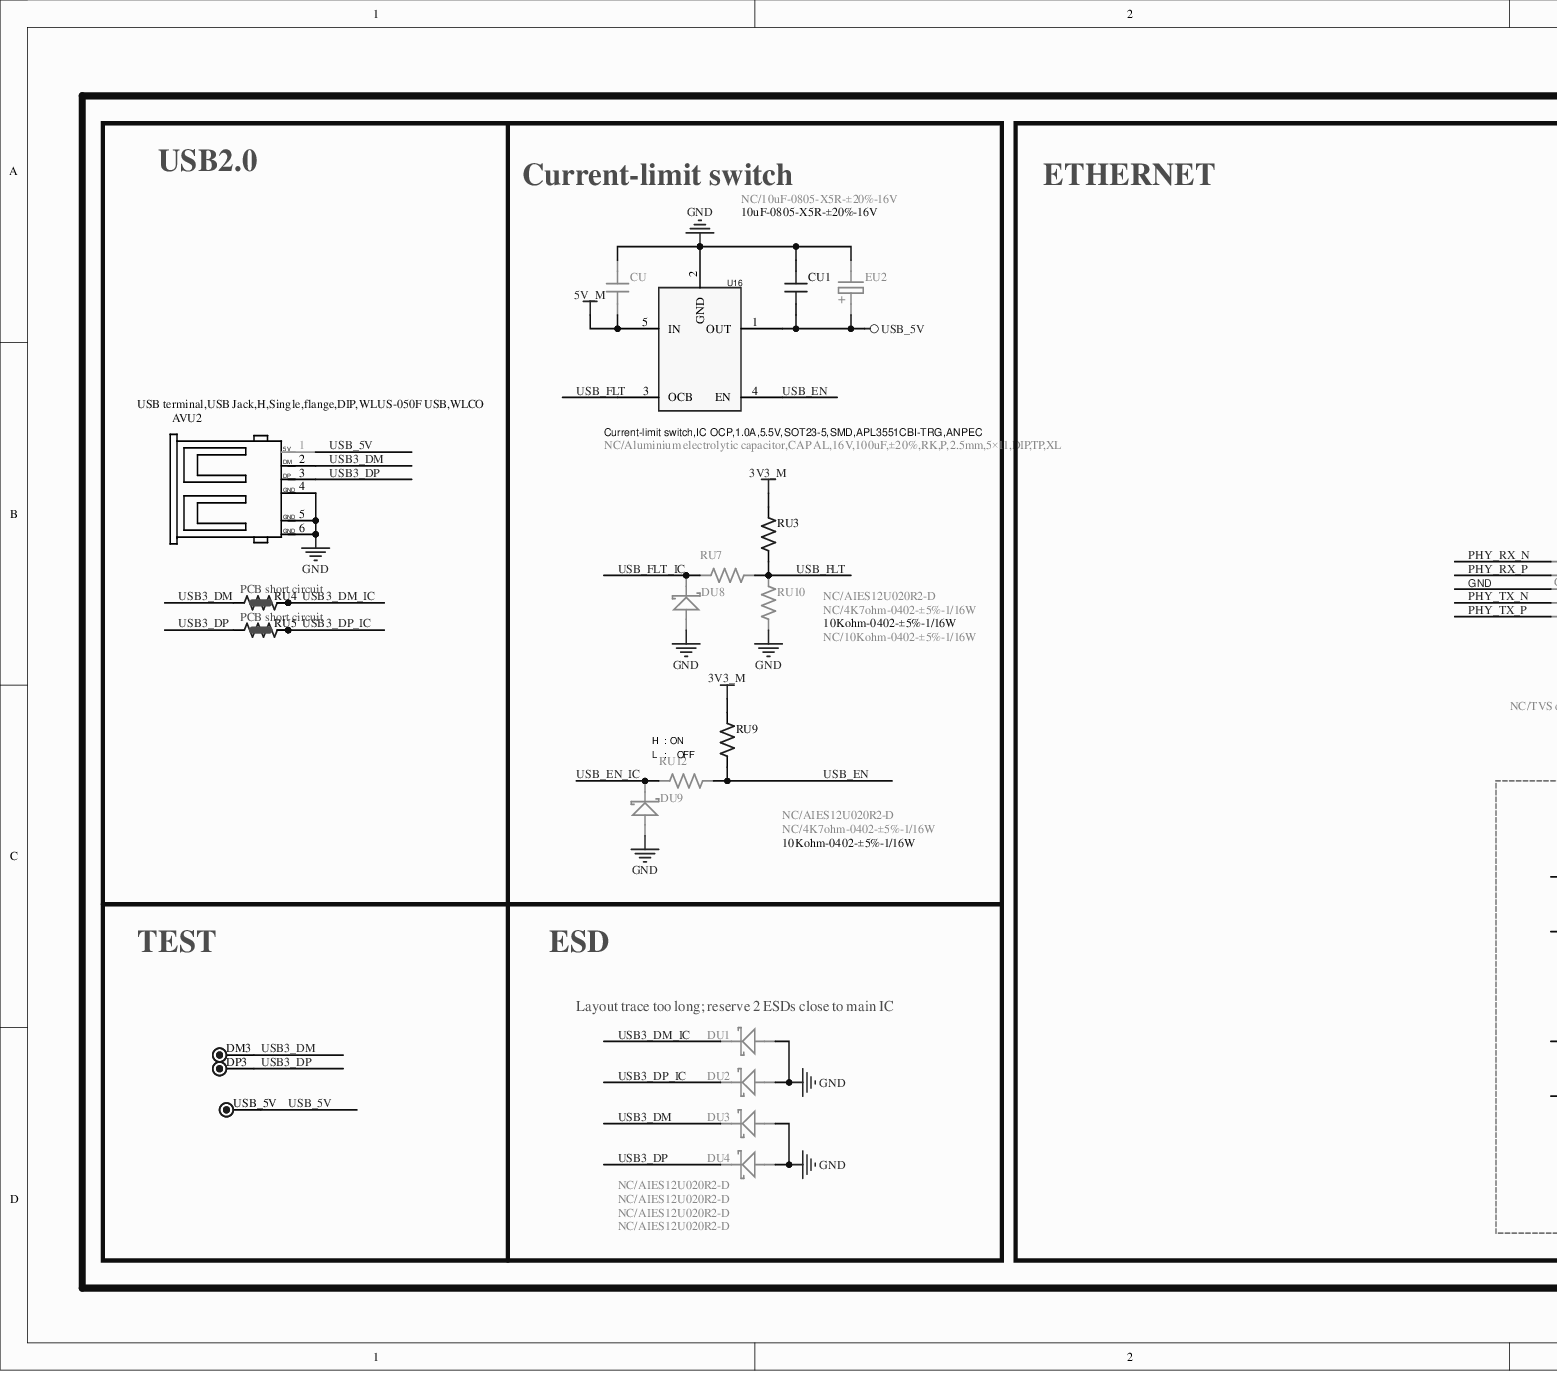
[diagram p0: MISC84395-14.SchDoc, left]
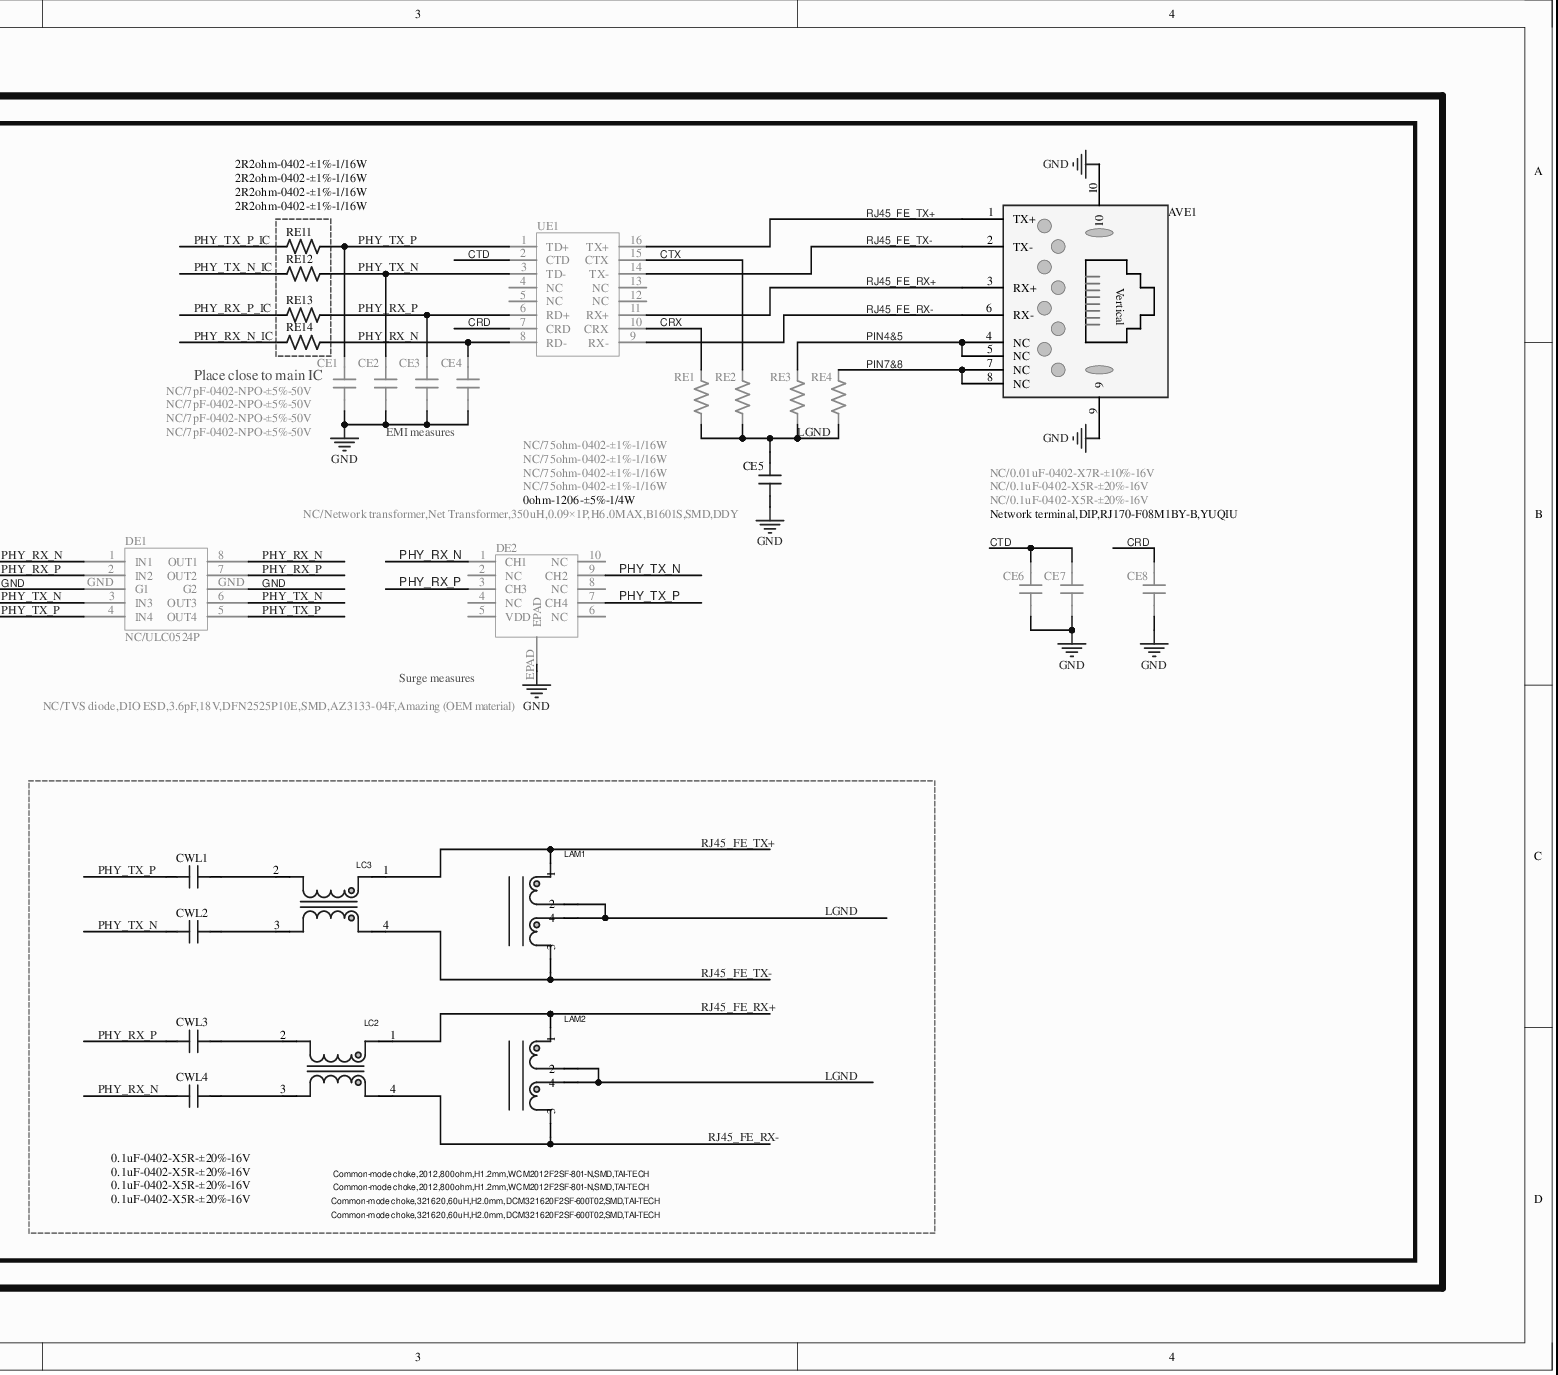
[diagram p1: MISC84395-14.SchDoc, right]
# Altium project MISC84395-37.PrjPCB (part 9 of 13)

## Sheet MISC84395-14.SchDoc
size 558 x 254 mm

### Parts
AVE1  Network terminal,DIP,RJ170-F08M1BY-B,YUQIU  [RJ45-VD-16]
AVU2  USB terminal,USB Jack,H,Single,flange,DIP,WLUS-050F USB,WLCO  [USB1-HD-2]
CE1  NC/7pF-0402-NPO-±5%-50V  [C0402]
CE2  NC/7pF-0402-NPO-±5%-50V  [C0402]
CE3  NC/7pF-0402-NPO-±5%-50V  [C0402]
CE4  NC/7pF-0402-NPO-±5%-50V  [C0402]
CE5  0ohm-1206-±5%-1/4W  [C1206]
CE6  NC/0.1uF-0402-X5R-±20%-16V  [C0402]
CE7  NC/0.01uF-0402-X7R-±10%-16V  [C0402]
CE8  NC/0.1uF-0402-X5R-±20%-16V  [C0402]
CU  NC/10uF-0805-X5R-±20%-16V  [C0805]
CU1  10uF-0805-X5R-±20%-16V  [C0805]
CWL1  0.1uF-0402-X5R-±20%-16V  [C0402]
CWL2  0.1uF-0402-X5R-±20%-16V  [C0402]
CWL3  0.1uF-0402-X5R-±20%-16V  [C0402]
CWL4  0.1uF-0402-X5R-±20%-16V  [C0402]
DE1  NC/ULC0524P  [RCL0524P]
DE2  NC/TVS diode,DIO ESD,3.6pF,18V,DFN2525P10E,SMD,AZ3133-04F,Amazing (OEM material)  [DFN10/0.5-2]
DM3  TEST  [TP]  (value not drawn)
DP3  TEST  [TP]  (value not drawn)
DU1  NC/AIES12U020R2-D  [DIODE-S0402]
DU2  NC/AIES12U020R2-D  [DIODE-S0402]
DU3  NC/AIES12U020R2-D  [DIODE-S0402]
DU4  NC/AIES12U020R2-D  [DIODE-S0402]
DU8  NC/AIES12U020R2-D  [DIODE-S0402]
DU9  NC/AIES12U020R2-D  [DIODE-S0402]
EU2  NC/Aluminium electrolytic capacitor,CAP AL,16V,100uF,±20%,RK,P,2.5mm,5×11,DIP,TP,XL  [EC(5*11)-V-2.5]
LAM1  Common-mode choke,321620,60uH,H2.0mm,DCM321620F2SF-600T02,SMD,TAI-TECH  [L/LC4/3.2*1.6]
LAM2  Common-mode choke,321620,60uH,H2.0mm,DCM321620F2SF-600T02,SMD,TAI-TECH  [L/LC4/3.2*1.6]
LC2  Common-mode choke,2012,800ohm,H1.2mm,WCM2012F2SF-801-N,SMD,TAI-TECH  [L/LC4/2*1.2-S]
LC3  Common-mode choke,2012,800ohm,H1.2mm,WCM2012F2SF-801-N,SMD,TAI-TECH  [L/LC4/2*1.2-S]
RE1  NC/75ohm-0402-±1%-1/16W  [R0402]
RE2  NC/75ohm-0402-±1%-1/16W  [R0402]
RE3  NC/75ohm-0402-±1%-1/16W  [R0402]
RE4  NC/75ohm-0402-±1%-1/16W  [R0402]
RE11  2R2ohm-0402-±1%-1/16W  [R0402]
RE12  2R2ohm-0402-±1%-1/16W  [R0402]
RE13  2R2ohm-0402-±1%-1/16W  [R0402]
RE14  2R2ohm-0402-±1%-1/16W  [R0402]
RU3  10Kohm-0402-±5%-1/16W  [R0402]
RU4  NC/0ohm-0402-PCB  [R0402SC]  (value not drawn)
RU5  NC/0ohm-0402-PCB  [R0402SC]  (value not drawn)
RU7  NC/4K7ohm-0402-±5%-1/16W  [R0402]
RU9  10Kohm-0402-±5%-1/16W  [R0402]
RU10  NC/10Kohm-0402-±5%-1/16W  [R0402]
RU12  NC/4K7ohm-0402-±5%-1/16W  [R0402]
U16  Current-limit switch,IC OCP,1.0A,5.5V,SOT23-5,SMD,APL3551CBI-TRG,ANPEC  [SOT-23-5]
UE1  NC/Network transformer,Net Transformer,350uH,0.09×1P,H6.0MAX,B1601S,SMD,DDY  [SOP16/1.27-2]
USB_5V  TEST  [TP]  (value not drawn)

### Blocks framed on the sheet
ETHERNET: AVE1 CE1-CE8 CWL1-CWL4 DE1 DE2 LAM1 LAM2 LC2 LC3 RE1-RE4 RE11-RE14 UE1

### Nets
3V3_M: RU3.2 RU9.2
5V_M: CU.1 U16.5(IN)
GND: AVE1.9 AVE1.10 AVU2.4 AVU2.5 AVU2.6 CE1.1 CE2.1 CE3.1 CE4.1 CE5.2 CE6.1 CE7.1 CE8.2 CU.2 CU1.1 DE1.GND(G1) DE2.EPAD DU1.A DU2.A DU3.A DU4.A DU8.A DU9.A EU2.2 RU10.1 U16.2(GND)
USB_5V: AVU2.1 CU1.2 EU2.1 U16.1(OUT) USB_5V.1
CRD: CE8.1 UE1.7(CRD)
CRX: RE1.2 UE1.10(CRX)
CTD: CE6.2 CE7.2 UE1.2(CTD)
CTX: RE2.2 UE1.15(CTX)
LGND: CE5.1 LAM1.2 LAM1.4 LAM2.2 LAM2.4 RE1.1 RE2.1 RE3.1 RE4.1
PHY_RX_N: CE4.2 CWL4.1 DE1.1(IN1) DE1.8(OUT1) DE2.1(CH1) RE14.2 UE1.8(RD-)
PHY_RX_N_IC: RE14.1
PHY_RX_P: CE3.2 CWL3.1 DE1.2(IN2) DE1.7(OUT2) DE2.3(CH3) RE13.2 UE1.6(RD+)
PHY_RX_P_IC: RE13.1
PHY_TX_N: CE2.2 CWL2.1 DE1.3(IN3) DE1.6(OUT3) DE2.9(CH2) RE12.2 UE1.3(TD-)
PHY_TX_N_IC: RE12.1
PHY_TX_P: CE1.2 CWL1.1 DE1.4(IN4) DE1.5(OUT4) DE2.7(CH4) RE11.2 UE1.1(TD+)
PHY_TX_P_IC: RE11.1
PIN4&5: AVE1.4(NC) AVE1.5(NC) RE3.2
PIN7&8: AVE1.7(NC) AVE1.8(NC) RE4.2
RJ45_FE_RX+: AVE1.3(RX+) LAM2.1 LC2.1 UE1.11(RX+)
RJ45_FE_RX-: AVE1.6(RX-) LAM2.3 LC2.4 UE1.9(RX-)
RJ45_FE_TX+: AVE1.1(TX+) LAM1.1 LC3.1 UE1.16(TX+)
RJ45_FE_TX-: AVE1.2(TX-) LAM1.3 LC3.4 UE1.14(TX-)
USB3_DM: AVU2.2 DM3.1 DU3.K RU4.1
USB3_DM_IC: DU1.K RU4.2 RU4.3
USB3_DP: AVU2.3 DP3.1 DU4.K RU5.1
USB3_DP_IC: DU2.K RU5.2 RU5.3
USB_EN: RU9.1 RU12.2 U16.4(EN)
USB_EN_IC: DU9.K RU12.1
USB_FLT: RU3.1 RU7.2 RU10.2 U16.3(OCB)
USB_FLT_IC: DU8.K RU7.1
NetCWL1_2: CWL1.2 LC3.2
NetCWL2_2: CWL2.2 LC3.3
NetCWL3_2: CWL3.2 LC2.2
NetCWL4_2: CWL4.2 LC2.3

Not connected (* = marked no-connect by the designer): DE2 2(NC)* 4(NC)* 5(VDD)* 6(NC)* 8(NC)* 10(NC)*; UE1 4(NC)* 5(NC)* 12(NC)* 13(NC)*

### Notes on the sheet
- USB2.0
- Current-limit switch
- (near CE1) Place close to main IC
- EMI measures
- (near DE2) Surge measures
- H :ON
- L : OFF
- TEST
- ESD
- (near DU1) Layout trace too long; reserve 2 ESDs close to main IC

### Library data of the parts
AVE1 = XXX.XXX.0004736-DHMI: Network terminal,DIP,RJ170-F08M1BY-B,YUQIU-DHMI
AVU2 = USB-2035A01-DHMI-USB: CN-USB-#-#-#
CE1-CE4 = 7pF-0402-NPO-±5%-50V-D
CE5 = 1000pF-1206-X7R-±20%-2000V-D
CE6 CE8 CWL1-CWL4 = 0.1uF-0402-X5R-±20%-16V-D
CE7 = 0.01uF-0402-X7R-±10%-16V-D
CU CU1 = 10uF-0805-X5R-+15%-16V-D
DE1 = RCLAMP0524P-TCT-D: RCLAMP0524J
DE2 = TVS管,DIO ESD,3.6pF,18V,DFN2525P10E,SMD,AZ3133-04F,Amazing（OEM物料）-D
DU1-DU4 DU8 DU9 = AIES12U020R2-D
EU2 = 100uF-16V-±20%-5×11-105℃-黑底白字-编带-F=2.5-XF-DHAI: Electrolytic
LAM1 LAM2 = PKG-003494/P000077171: Common-mode choke,60uH,2.0mm,SMD,sunlord-D
LC2 LC3 = 004.004.0002112: Common-mode choke,2012,800Ω,1.2mm,WCM2012F2SF-801-N,SMD,TAI-TECH-D
RE1-RE4 = 75ohm-0402-±1%-1/16W-D
RE11-RE14 = 2R2ohm-0402-±1%-1/16W-D
RU3 RU7 RU9 RU10 RU12 = 4K7ohm-0402-±5%-1/16W-D
RU4 RU5 = 0ohm-0402-PCB-D
U16 = 限流开关,IC OCP,1.0A,5.5V,SOT-23-5,SMD,APL3551CBI-TRG,ANPEC-D
UE1 = H16101MC-D

## Sheet MISC84395-15.SchDoc
size 203 x 279 mm
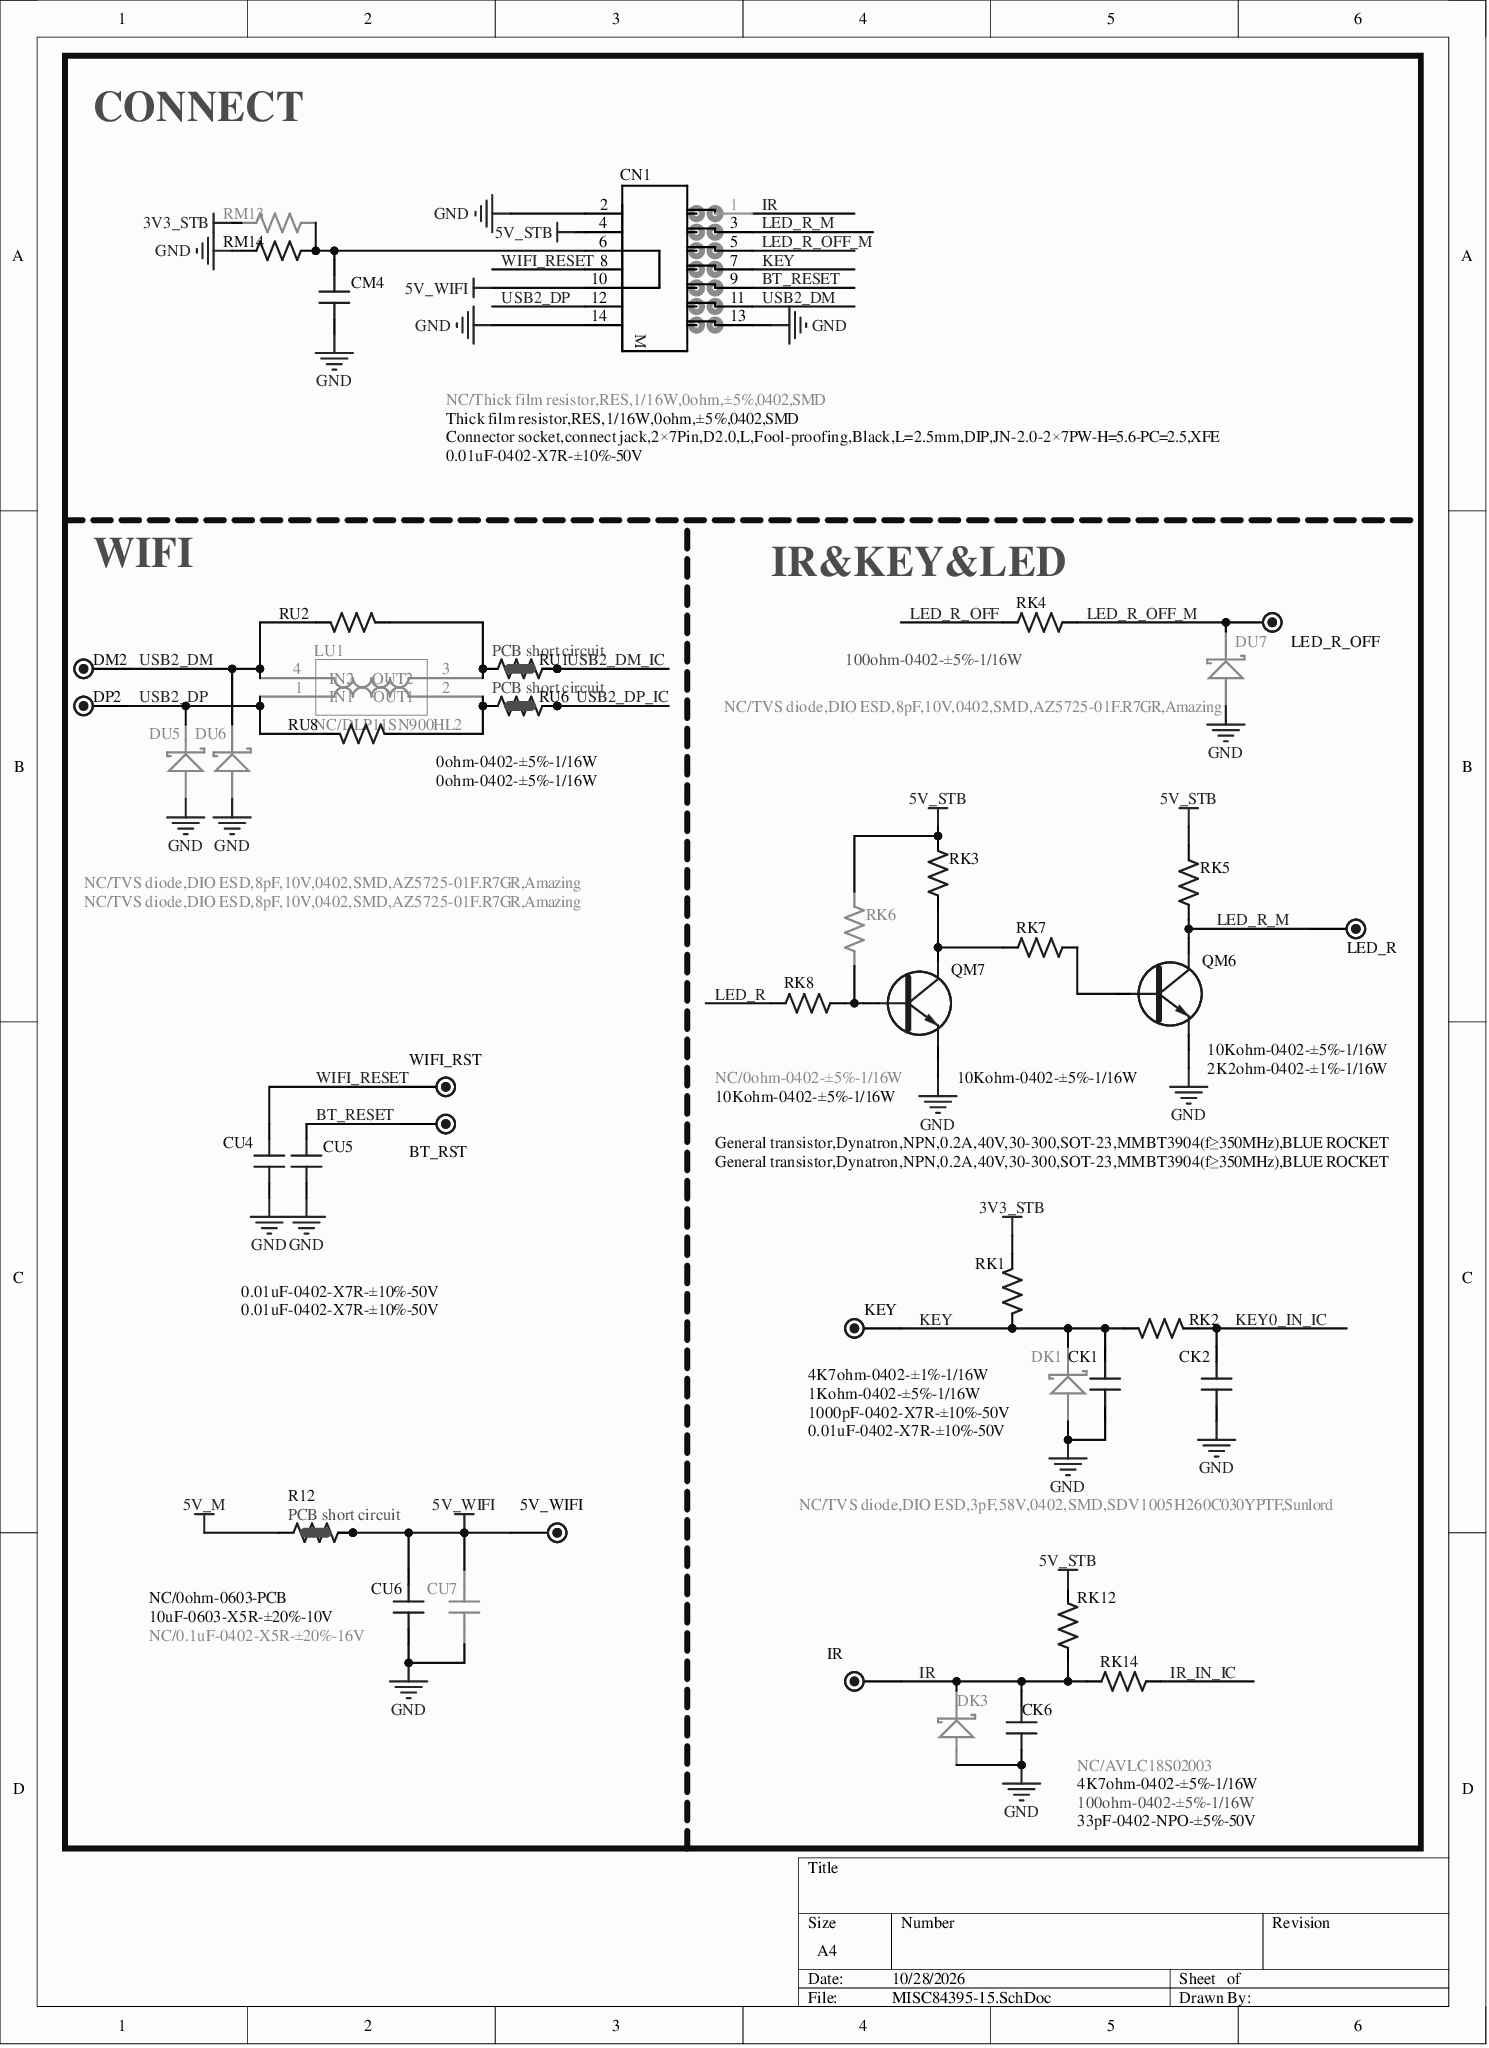
[diagram p2: MISC84395-15.SchDoc]

### Parts
5V_WIFI  TEST  [TP]  (value not drawn)
BT_RST  TEST  [TP]  (value not drawn)
CK1  1000pF-0402-X7R-±10%-50V  [C0402]
CK2  0.01uF-0402-X7R-±10%-50V  [C0402]
CK6  33pF-0402-NPO-±5%-50V  [C0402]
CM4  0.01uF-0402-X7R-±10%-50V  [C0402]
CN1  Connector socket,connect jack,2×7Pin,D2.0,L,Fool-proofing,Black,L=2.5mm,DIP,JN-2.0-2×7PW-H=5.6-PC=2.5,XFE  [SIP2*7H/2.0DM-8]
CU4  0.01uF-0402-X7R-±10%-50V  [C0402]
CU5  0.01uF-0402-X7R-±10%-50V  [C0402]
CU6  10uF-0603-X5R-±20%-10V  [C0603]
CU7  NC/0.1uF-0402-X5R-±20%-16V  [C0402]
DK1  NC/TVS diode,DIO ESD,3pF,58V,0402,SMD,SDV1005H260C030YPTF,Sunlord  [DIODE-S0402]
DK3  NC/AVLC18S02003  [DIODE-S0402]
DM2  TEST  [TP]  (value not drawn)
DP2  TEST  [TP]  (value not drawn)
DU5  NC/TVS diode,DIO ESD,8pF,10V,0402,SMD,AZ5725-01F.R7GR,Amazing  [DIODE-S0402]
DU6  NC/TVS diode,DIO ESD,8pF,10V,0402,SMD,AZ5725-01F.R7GR,Amazing  [DIODE-S0402]
DU7  NC/TVS diode,DIO ESD,8pF,10V,0402,SMD,AZ5725-01F.R7GR,Amazing  [DIODE-S0402]
IR  TEST  [TP]  (value not drawn)
KEY  TEST  [TP]  (value not drawn)
LED_R  TEST  [TP]  (value not drawn)
LED_R_OFF  TEST  [TP]  (value not drawn)
LU1  NC/DLP11SN900HL2  [L/LC4/1.25*1.0]
QM6  General transistor,Dynatron,NPN,0.2A,40V,30-300,SOT-23,MMBT3904(f≥350MHz),BLUE ROCKET  [SOT-23]
QM7  General transistor,Dynatron,NPN,0.2A,40V,30-300,SOT-23,MMBT3904(f≥350MHz),BLUE ROCKET  [SOT-23]
R12  NC/0ohm-0603-PCB  [R0603SC]
RK1  4K7ohm-0402-±1%-1/16W  [R0402]
RK2  1Kohm-0402-±5%-1/16W  [R0402]
RK3  10Kohm-0402-±5%-1/16W  [R0402]
RK4  100ohm-0402-±5%-1/16W  [R0402]
RK5  2K2ohm-0402-±1%-1/16W  [R0402]
RK6  NC/0ohm-0402-±5%-1/16W  [R0402]
RK7  10Kohm-0402-±5%-1/16W  [R0402]
RK8  10Kohm-0402-±5%-1/16W  [R0402]
RK12  4K7ohm-0402-±5%-1/16W  [R0402]
RK14  100ohm-0402-±5%-1/16W  [R0402]
RM13  NC/Thick film resistor,RES,1/16W,0ohm,±5%,0402,SMD  [R0402]
RM14  Thick film resistor,RES,1/16W,0ohm,±5%,0402,SMD  [R0402]
RU1  NC/0ohm-0402-PCB  [R0402SC]  (value not drawn)
RU2  0ohm-0402-±5%-1/16W  [R0402]
RU6  NC/0ohm-0402-PCB  [R0402SC]  (value not drawn)
RU8  0ohm-0402-±5%-1/16W  [R0402]
WIFI_RST  TEST  [TP]  (value not drawn)

### Nets
3V3_STB: RK1.2 RM13.2
5V_M: R12.1
5V_STB: CN1.4 RK3.2 RK5.1 RK6.2 RK12.2
5V_WIFI: 5V_WIFI.1 CN1.10 CU6.1 CU7.1 R12.2 R12.3
GND: CK1.2 CK2.2 CK6.1 CM4.1 CN1.2 CN1.13 CN1.14 CU4.1 CU5.1 CU6.2 CU7.2 DK1.A DK3.A DU5.A DU6.A DU7.A QM6.E QM7.E RM14.2
BT_RESET: BT_RST.1 CN1.9 CU5.2
IR: CK6.2 CN1.1 DK3.K IR.1 RK12.1 RK14.1
IR_IN_IC: RK14.2
KEY: CK1.1 CN1.7 DK1.K KEY.1 RK1.1 RK2.2
KEY0_IN_IC: CK2.1 RK2.1
LED_R: RK8.1
LED_R_M: CN1.3 LED_R.1 QM6.C RK5.2
LED_R_OFF: RK4.1
LED_R_OFF_M: CN1.5 DU7.K LED_R_OFF.1 RK4.2
USB2_DM: CN1.11 DM2.1 DU6.K LU1.4(IN2) RU2.1
USB2_DM_IC: RU1.2 RU1.3
USB2_DP: CN1.12 DP2.1 DU5.K LU1.1(IN1) RU8.1
USB2_DP_IC: RU6.2 RU6.3
WIFI_RESET: CN1.8 CU4.2 WIFI_RST.1
NetCM4_2: CM4.2 CN1.6 RM13.1 RM14.1
NetLU1_2: LU1.2(OUT1) RU6.1 RU8.2
NetLU1_3: LU1.3(OUT2) RU1.1 RU2.2
NetQM6_B: QM6.B RK7.1
NetQM7_B: QM7.B RK6.1 RK8.2
NetQM7_C: QM7.C RK3.1 RK7.2

### Notes on the sheet
- CONNECT
- WIFI
- (near RK4) IR&KEY&LED

### Library data of the parts
CK1 CK2 CM4 CU4 CU5 = 0.01uF-0402-X7R-±10%-50V-D
CK6 = 22pF-0402-NPO-±5%-50V-D
CN1 = XXX.XXX.0004726-DLMI
CU6 = 10uF-0603-X5R-±20%-6.3V-D
CU7 = 0.1uF-0402-X5R-±20%-16V-D
DK1 = SFI0402-240E-2R5PP-LF-D
DK3 = AVLC18S02003-D
DU5-DU7 = AIES12U020R2-D
LU1 = DLP11SN900HL2-D: CHOKE COIL COMMON MODE 100MA Z0=90ohm
QM6 QM7 = KMBT3904-D
R12 = 0ohm-0603-PCB-D
RK1 = 4K7ohm-0402-±1%-1/16W-D
RK2 = 1Kohm-0402-±5%-1/16W-D
RK3 RK5-RK8 = 10Kohm-0402-±5%-1/16W-D
RK4 RK14 = 100ohm-0402-±5%-1/16W-D
RK12 = 4K7ohm-0402-±5%-1/16W-D
RM13 RM14 = 004.002.0000558-D: Thick film resistor,RES,1/16W,0ohm,±5%,0402,SMD-D
RU1 RU6 = 0ohm-0402-PCB-D
RU2 RU8 = 5R1ohm-0402-±5%-1/16W-D